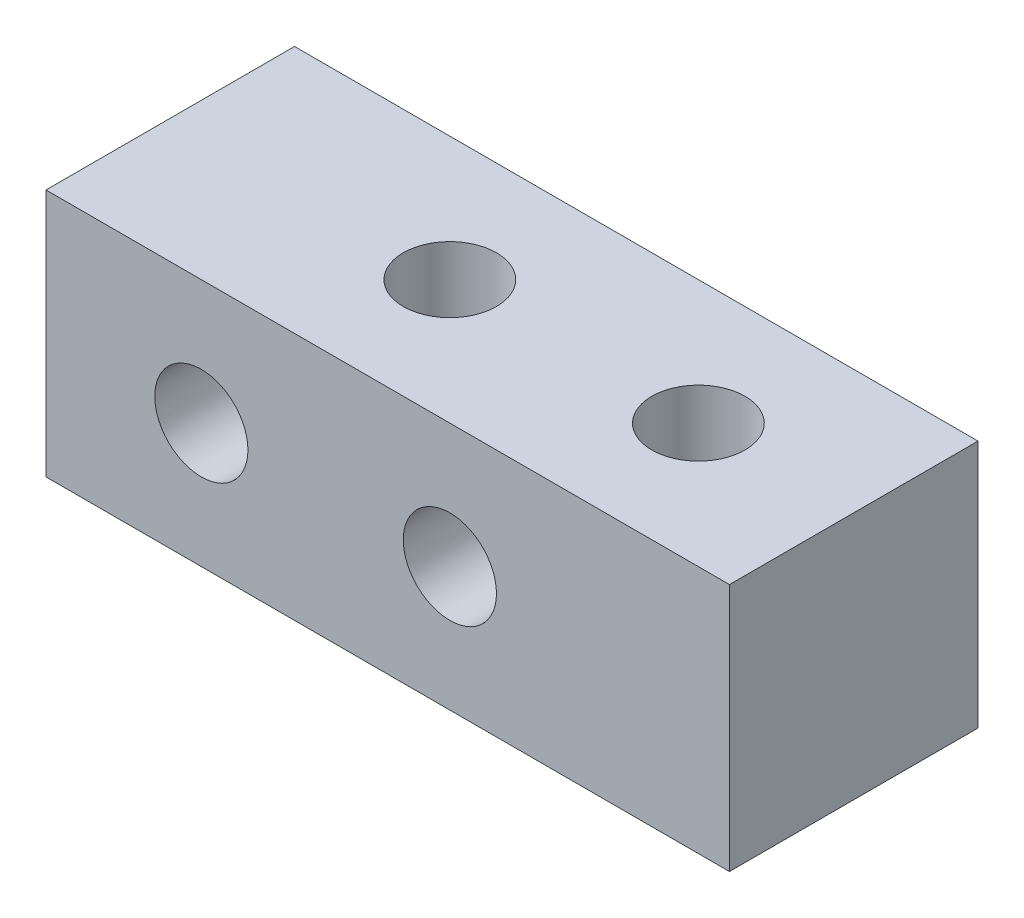
SolidWorks part; units mm, degrees
other "标注1"
sketch "草图3" plane through (-11, 4, 8) normal (-0.3003, 0.938, 0.1731) x (0.9538, 0.2931, 0.0666)
material "6061 合金"
ref_plane "前视基准面" through (0, 0, 0) normal (0, 0, 1) x (1, 0, 0)
ref_plane "上视基准面" through (0, 0, 0) normal (0, 1, 0) x (1, 0, 0)
ref_plane "右视基准面" through (0, 0, 0) normal (1, 0, 0) x (0, 0, -1)
sketch "草图1" plane through (0, 0, 0) normal (0, 0, 1) x (1, 0, 0)
  line L0 (0, 0) -> (-6, 0) construction
  line L1 (11, 4) -> (-11, 4)
  line L2 (11, 4) -> (11, -4)
  line L3 (11, -4) -> (-11, -4)
  line L4 (-11, 4) -> (-11, -4)
  line L5 (11, 4) -> (-11, -4) construction
  line L6 (11, -4) -> (-11, 4) construction
  line L7 (0, 0) -> (2, 0) construction
  circle A0 centre (-6, 0) radius 1.5
  circle A1 centre (2, 0) radius 1.5
  point P0 (0, 0)
  dimension "D3" = 3
  dimension "D1" = 22
  dimension "D2" = 8
  dimension "D4" = 8
  dimension "D5" = 5
extrude "凸台-拉伸1" add sketch "草图1" along normal blind 8
sketch "草图2" plane through (0, 4, 0) normal (0, 1, 0) x (1, 0, 0)
  line L0 (0, 0) -> (0, -4) construction
  line L1 (0, -4) -> (11, -4) construction
  line L2 (11, -8) -> (11, 0) construction
  circle A0 centre (6, -4) radius 1.5
  circle A1 centre (-2, -4) radius 1.5
  dimension "D1" = 5
  dimension "D3" = 3
  dimension "D2" = 8
extrude "切除-拉伸1" cut sketch "草图2" against normal through all
